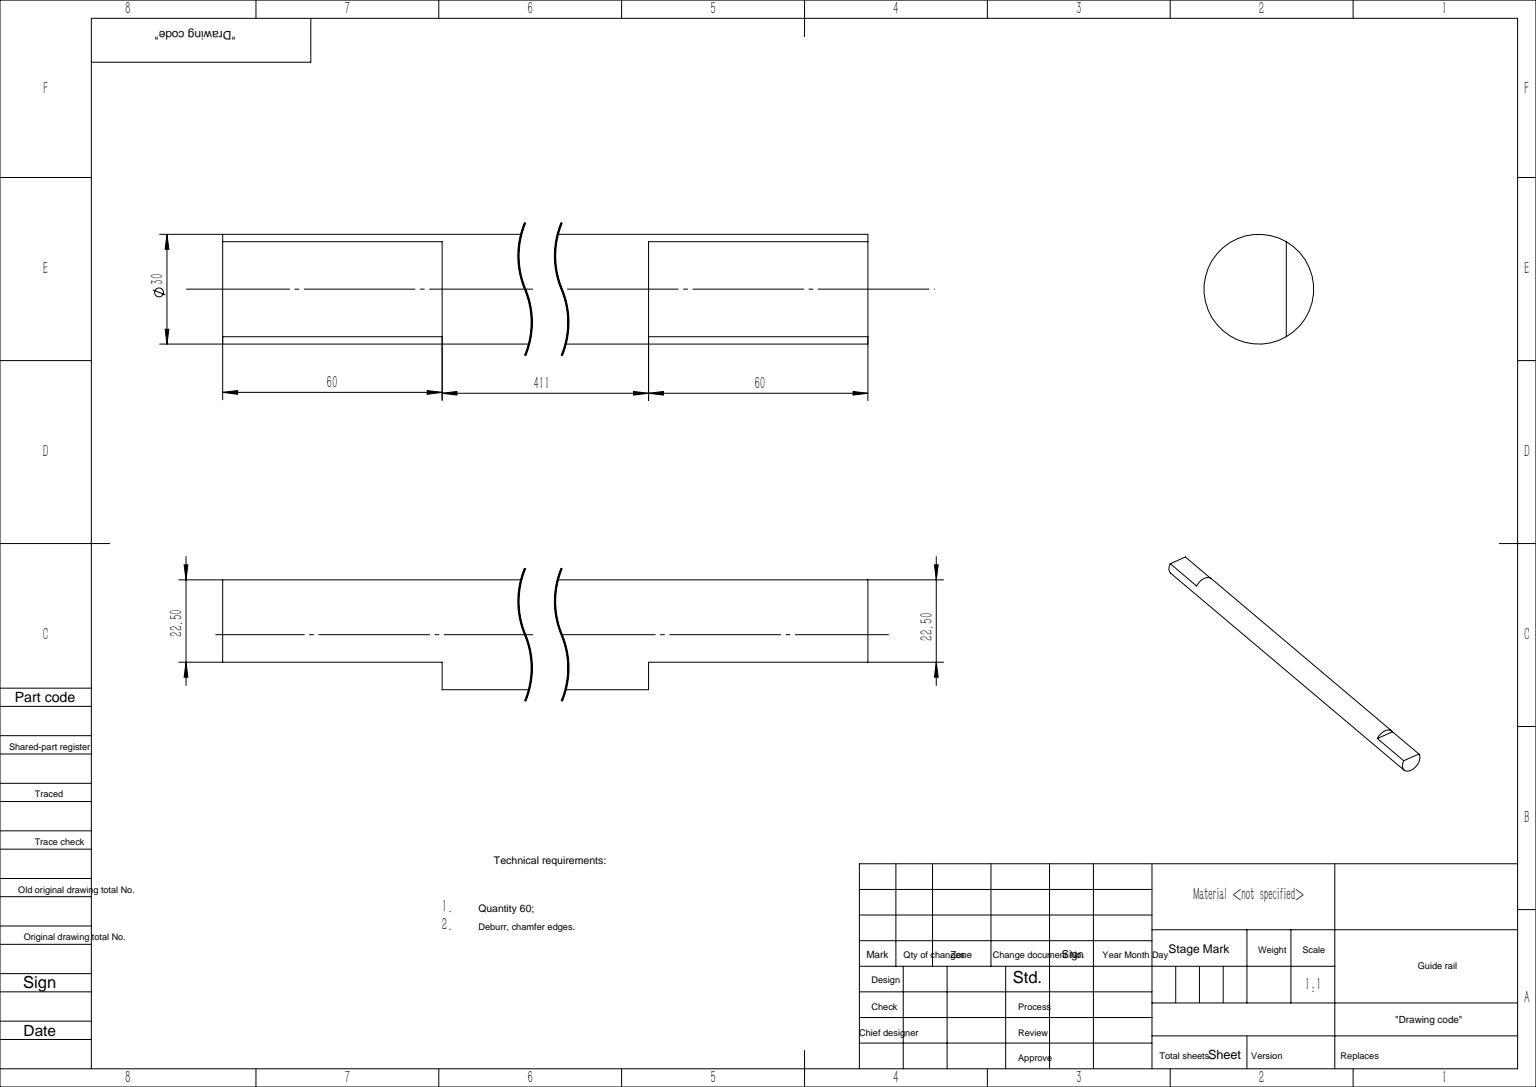
from build123d import *

# Parameters (mm, degrees)
SKETCH_1_R          = 15
EXTRUDE_1_DEPTH     = 531
CUT_EXTRUDE_START   = -60
CUT_EXTRUDE_1_DEPTH = 60


with BuildPart() as part:
    # 草图1 → 凸台-拉伸1 (new body)
    with BuildSketch(Plane(origin=(0, 0, 0), x_dir=(1, 0, 0), z_dir=(0, 1, 0))):
        with Locations(Location((0, 0, 0), (0, 0, 270))):
            Circle(SKETCH_1_R)
    extrude(amount=EXTRUDE_1_DEPTH)

    # 草图2 → 切除-拉伸1 (cut)
    with BuildSketch(Plane(origin=(0, 531, 0), x_dir=(1, 0, 0), z_dir=(0, 1, 0)).offset(CUT_EXTRUDE_START)):
        with BuildLine():
            Line((7.5, 12.990381057), (7.5, -12.990381057))
            ThreePointArc((7.5, -12.990381057), (15, 0), (7.5, 12.990381057))
        make_face()
    cut_extrude_1 = extrude(amount=CUT_EXTRUDE_1_DEPTH, mode=Mode.SUBTRACT)

    # 镜向1: 切除-拉伸1 across plane
    add(cut_extrude_1.mirror(Plane.ZX.offset(265.5)), mode=Mode.SUBTRACT)


solid = part.part
